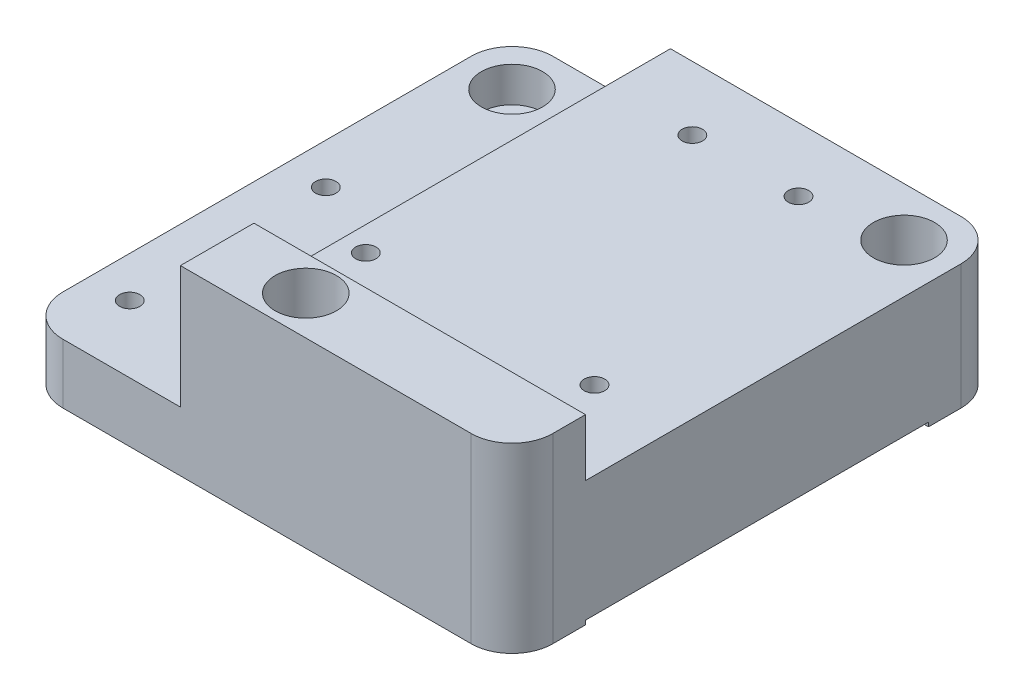
from build123d import *

# Parameters (mm, degrees)
SKETCH_1_3_W          = 40.6
SKETCH_1_3_H          = 60
BOSS_EXTRUDE1_DEPTH   = 15.3
SKETCH_1_3_2_W        = 19.4
SKETCH_1_3_2_H        = 60
BOSS_EXTRUDE2_DEPTH   = 7.3
SKETCH2_W             = 40.6
SKETCH2_H             = 9
BOSS_EXTRUDE3_DEPTH   = 7
M3_TAPPED_HOLE1_D     = 2.5
M3_TAPPED_HOLE1_DEPTH = 7.5
M3_TAPPED_HOLE1_TIP   = 0.751075774
M3_TAPPED_HOLE2_D     = 2.5
M3_TAPPED_HOLE2_DEPTH = 7.5
M3_TAPPED_HOLE2_TIP   = 0.751075774
FILLET1_R             = 5
SKETCH11_W            = 42
SKETCH11_H            = 4.723838164
CUT_EXTRUDE5_DEPTH    = 73.78462902
SKETCH12_R            = 3.75
CUT_EXTRUDE6_DEPTH    = 19.3
SKETCH13_R            = 2.2
CUT_EXTRUDE7_DEPTH    = 52.321618612


with BuildPart() as part:
    # Sketch 1_3 → Boss-Extrude1 (new body)
    with BuildSketch(Plane(origin=(0, 0, 0), x_dir=(1, 0, 0), z_dir=(0, 1, 0))):
        with Locations((7.125373134, -4.645522388)):
            Rectangle(SKETCH_1_3_W, SKETCH_1_3_H)
    extrude(amount=BOSS_EXTRUDE1_DEPTH)

    # Sketch 1_3 2 → Boss-Extrude2 (add)
    with BuildSketch(Plane(origin=(0, 0, 0), x_dir=(1, 0, 0), z_dir=(0, 1, 0))):
        with Locations((-22.874626866, -4.645522388)):
            Rectangle(SKETCH_1_3_2_W, SKETCH_1_3_2_H)
    extrude(amount=BOSS_EXTRUDE2_DEPTH)

    # Sketch2 → Boss-Extrude3 (add)
    with BuildSketch(Plane(origin=(0, 15.3, 0), x_dir=(1, 0, 0), z_dir=(0, 1, 0))):
        with Locations((7.125373134, -30.145522388)):
            Rectangle(SKETCH2_W, SKETCH2_H)
    extrude(amount=BOSS_EXTRUDE3_DEPTH)

    # M3 Tapped Hole1
    with Locations(Plane(origin=(0, 7.3, 0), x_dir=(1, 0, 0), z_dir=(0, 1, 0))):
        with Locations((-27.574626866, -2.445522388), (-27.574626866, -26.445522388)):
            Hole(M3_TAPPED_HOLE1_D / 2, depth=M3_TAPPED_HOLE1_DEPTH)
            with Locations((0, 0, -(M3_TAPPED_HOLE1_DEPTH + M3_TAPPED_HOLE1_TIP / 2))):  # 118° drill point
                Cone(0, M3_TAPPED_HOLE1_D / 2, M3_TAPPED_HOLE1_TIP, mode=Mode.SUBTRACT)

    # M3 Tapped Hole2
    with Locations(Plane(origin=(0, 15.3, 0), x_dir=(1, 0, 0), z_dir=(0, 1, 0))):
        with Locations((-10.174626866, -14.945522388), (17.825373134, -14.945522388), (-2.674626866, 17.534477612), (10.325373134, 17.534477612)):
            Hole(M3_TAPPED_HOLE2_D / 2, depth=M3_TAPPED_HOLE2_DEPTH)
            with Locations((0, 0, -(M3_TAPPED_HOLE2_DEPTH + M3_TAPPED_HOLE2_TIP / 2))):  # 118° drill point
                Cone(0, M3_TAPPED_HOLE2_D / 2, M3_TAPPED_HOLE2_TIP, mode=Mode.SUBTRACT)

    # Fillet1
    fillet1_edges = [part.edges().sort_by_distance(p)[0] for p in [
        (-32.574626866, 3.65, -25.354477612),
        (-32.574626866, 3.65, 34.645522388),
        (27.425373134, 11.15, 34.645522388),
        (27.425373134, 7.65, -25.354477612),
    ]]
    fillet(fillet1_edges, radius=FILLET1_R)

    # Sketch11 → Cut-Extrude5 (cut, through all)
    with BuildSketch(Plane.ZY.offset(32.574626866)):
        with Locations((4.645522388, -1.861919082)):
            Rectangle(SKETCH11_W, SKETCH11_H)
    extrude(amount=-CUT_EXTRUDE5_DEPTH, mode=Mode.SUBTRACT)

    # Sketch12 → Cut-Extrude6 (cut)
    with BuildSketch(Plane(origin=(0, 22.3, 0), x_dir=(1, 0, 0), z_dir=(0, 1, 0))):
        with Locations(Location((21.425373134, 19.354477612, 0), (0, 0, 270))):
            Circle(SKETCH12_R)
        with Locations(Location((-26.574626866, 19.354477612, 0), (0, 0, 270))):
            Circle(SKETCH12_R)
        with Locations(Location((-2.574626866, -29.895522388, 0), (0, 0, 270))):
            Circle(SKETCH12_R)
    extrude(amount=-CUT_EXTRUDE6_DEPTH, mode=Mode.SUBTRACT)

    # Sketch13 → Cut-Extrude7 (cut, through all)
    with BuildSketch(Plane(origin=(0, 3, 0), x_dir=(1, 0, 0), z_dir=(0, 1, 0))):
        with Locations(Location((-2.574626866, -29.895522388, 0), (0, 0, 270))):
            Circle(SKETCH13_R)
        with Locations(Location((21.425373134, 19.354477612, 0), (0, 0, 270))):
            Circle(SKETCH13_R)
        with Locations(Location((-26.574626866, 19.354477612, 0), (0, 0, 270))):
            Circle(SKETCH13_R)
    extrude(amount=-CUT_EXTRUDE7_DEPTH, mode=Mode.SUBTRACT)


solid = part.part
